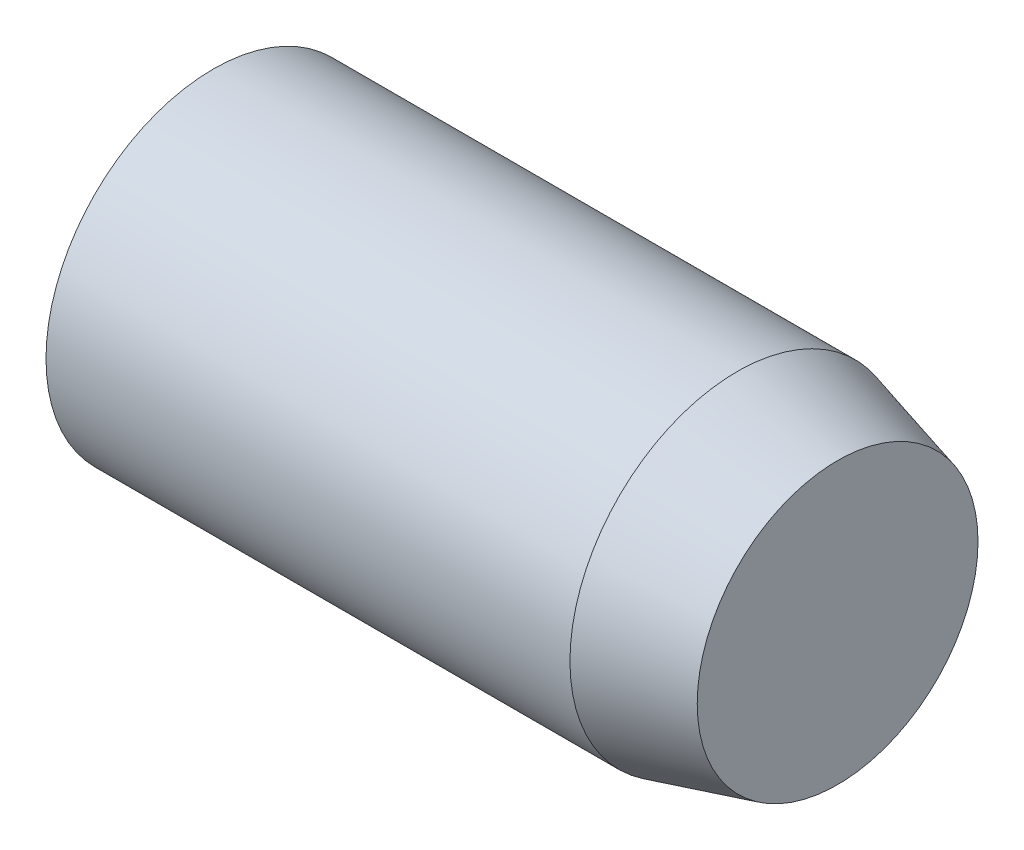
from build123d import *


with BuildPart() as part:
    # Sketch1 → Revolve1 (revolve)
    with BuildSketch(Plane(origin=(0, 0, 0), x_dir=(1, 0, 0), z_dir=(0, 1, 0))):
        with BuildLine():
            Line((-1.5, -2.5), (0, -2.098076211))
            Line((0, -2.098076211), (0, 0))
            Line((0, 0), (-10, 0))
            ThreePointArc((-10, 0), (-9.829629131, -1.294095226), (-9.330127019, -2.5))
            Line((-9.330127019, -2.5), (-1.5, -2.5))
        make_face()
    revolve(axis=Axis((-11.390713055, 0, 0), (1, 0, 0)))


solid = part.part
